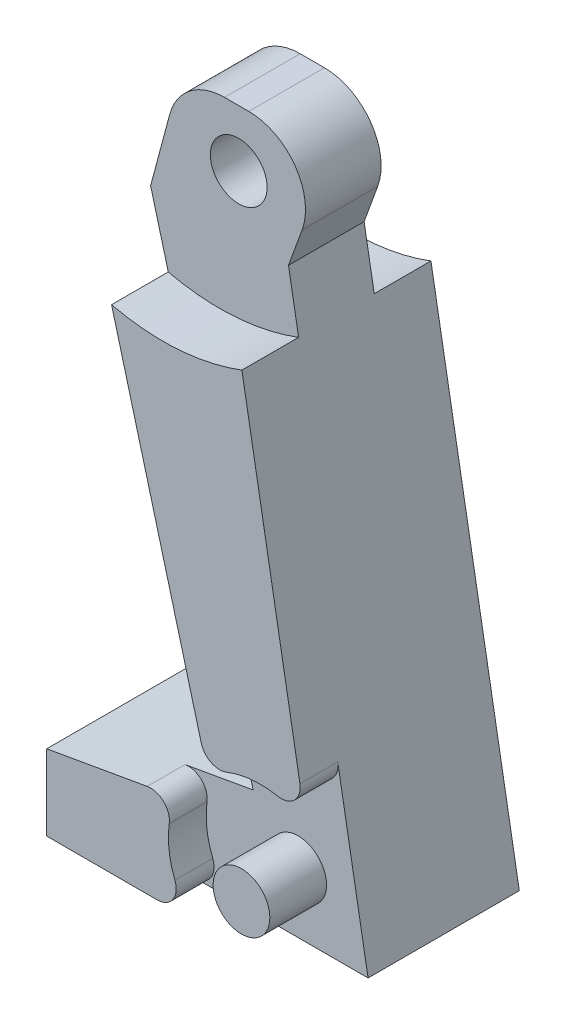
from build123d import *

# Parameters (mm, degrees)
BOSS_EXTRUDE1_DEPTH = 10
SKETCH2_W           = 14
SKETCH2_H           = 30
BOSS_EXTRUDE2_DEPTH = 30
BOSS_EXTRUDE4_DEPTH = 5
SKETCH5_W           = 6
SKETCH5_H           = 7
BOSS_EXTRUDE5_DEPTH = 6
SKETCH6_W           = 15
SKETCH6_H           = 15
BOSS_EXTRUDE6_DEPTH = 14
SKETCH7_R           = 1
CUT_EXTRUDE1_DEPTH  = 2
FILLET1_R           = 1
SKETCH8_R           = 1.5
SKETCH8_W           = 21.297654542
SKETCH8_H           = 29.54423259
CUT_EXTRUDE2_DEPTH  = 10
SKETCH9_W           = 4
SKETCH9_H           = 12
CUT_EXTRUDE3_DEPTH  = 7.5
SKETCH11_R          = 1.5
SKETCH11_W          = 46.682021109
SKETCH11_H          = 78.101327177
CUT_EXTRUDE6_DEPTH  = 50
SKETCH12_W          = 25.193851166
SKETCH12_H          = 16.960566472
CUT_EXTRUDE7_DEPTH  = 20
FILLET2_R           = 3
SKETCH13_W          = 3
SKETCH13_H          = 6
CUT_EXTRUDE8_DEPTH  = 20
SKETCH14_R          = 11.800022464
CUT_EXTRUDE9_DEPTH  = 3
SKETCH15_R          = 1.5
BOSS_EXTRUDE7_DEPTH = 1
SKETCH16_R          = 4.865347009
SKETCH16_R_2        = 1.5
CUT_EXTRUDE10_DEPTH = 2
FILLET5_R           = 1


with BuildPart() as part:
    # Sketch1 → Boss-Extrude1 (new body)
    with BuildSketch(Plane.XY):
        Polygon((0, 0), (15, 0), (9.79055467, 29.54423259), (20.05115897, 57.735011214), (10.05115897, 57.735011214), (2.497462604, 29.54423259), (8.920552671, 5.572934119), (0, 4), align=None)
    boss_extrude1 = extrude(amount=BOSS_EXTRUDE1_DEPTH)

    # Sketch2 → Boss-Extrude2 (add)
    with BuildSketch(Plane.XY.offset(10)):
        with Locations((15.05115897, 72.735011214)):
            Rectangle(SKETCH2_W, SKETCH2_H)
    extrude(amount=-BOSS_EXTRUDE2_DEPTH)

    # Sketch4 → Boss-Extrude4 (add)
    with BuildSketch(Plane.XY.offset(10)):
        Polygon((15.05115897, 84.235011214), (30.372047832, 71.37925902), (30.372047832, 56.37925902), (27.30787006, 56.37925902), (27.30787006, 68.950409459), (15.05115897, 79.235011214), align=None)
    boss_extrude4 = extrude(amount=BOSS_EXTRUDE4_DEPTH)

    # Mirror1: Boss-Extrude1, Boss-Extrude4 across plane
    add(boss_extrude1.mirror(Plane.XY.offset(-5)))
    add(boss_extrude4.mirror(Plane.XY.offset(-5)))

    # Sketch5 → Boss-Extrude5 (add)
    with BuildSketch(Plane(origin=(0, 87.735011214, 0), x_dir=(1, 0, 0), z_dir=(0, 1, 0))):
        with Locations((15.05115897, 5)):
            Rectangle(SKETCH5_W, SKETCH5_H)
    extrude(amount=BOSS_EXTRUDE5_DEPTH)

    # Sketch6 → Boss-Extrude6 (add)
    with BuildSketch(Plane(origin=(0, 93.735011214, 0), x_dir=(1, 0, 0), z_dir=(0, 1, 0))):
        with Locations((15.05115897, 5)):
            Rectangle(SKETCH6_W, SKETCH6_H)
    extrude(amount=BOSS_EXTRUDE6_DEPTH)

    # Sketch7 → Cut-Extrude1 (cut)
    with BuildSketch(Plane.ZY.offset(-7.55115897)):
        with Locations((-8.96, 103.735011214)):
            Circle(SKETCH7_R)
        with Locations(Location((-1.04, 103.735011214, 0), (0, 0, 180))):
            Circle(SKETCH7_R)
    extrude(amount=-CUT_EXTRUDE1_DEPTH, mode=Mode.SUBTRACT)

    # Fillet1
    fillet1_edges = [part.edges().sort_by_distance(p)[0] for p in [
        (18.55115897, 81.298162505, 10),
        (15.05115897, 81.735011214, 10),
        (15.05115897, 84.235011214, 12.5),
        (18.55115897, 76.298162505, 10),
        (15.05115897, 79.235011214, 12.5),
        (18.55115897, 81.298162505, -20),
        (18.55115897, 76.298162505, -20),
        (15.05115897, 81.735011214, -20),
        (15.05115897, 79.235011214, -22.5),
        (15.05115897, 84.235011214, -22.5),
    ]]
    fillet(fillet1_edges, radius=FILLET1_R)

    # Sketch8 → Cut-Extrude2 (cut)
    with BuildSketch(Plane(origin=(0, 0, -20), x_dir=(-1, 0, 0), z_dir=(0, 0, -1))):
        with Locations((-7.157843169, 32.54423259)):
            Circle(SKETCH8_R)
        with Locations((-4.351172729, 14.772116295)):
            Rectangle(SKETCH8_W, SKETCH8_H)
    extrude(amount=-CUT_EXTRUDE2_DEPTH, mode=Mode.SUBTRACT)

    # Sketch9 → Cut-Extrude3 (cut, symmetric)
    with BuildSketch(Plane.ZY.offset(-8.05115897)):
        with Locations((-15, 30.54423259)):
            Rectangle(SKETCH9_W, SKETCH9_H)
    extrude(amount=CUT_EXTRUDE3_DEPTH, both=True, mode=Mode.SUBTRACT)

    # Sketch11 → Cut-Extrude6 (cut, symmetric)
    with BuildSketch(Plane(origin=(0, 0, -20), x_dir=(-1, 0, 0), z_dir=(0, 0, -1))):
        with Locations(Location((-7.157843169, 32.54423259, 0), (0, 0, 180))):
            Circle(SKETCH11_R)
        with Locations((-27.446168312, 74.594896179)):
            Rectangle(SKETCH11_W, SKETCH11_H)
    extrude(amount=CUT_EXTRUDE6_DEPTH, both=True, mode=Mode.SUBTRACT)


with BuildPart() as cut_extrude6_piece_1:
    # of the separate pieces the step leaves, piece 1, a body of its own (cut_extrude6_pieces)
    add(part.part.solids().sort_by_distance((4.105157758, 35.54423259, 10))[0])

    # Fillet2
    fillet2_edges = [cut_extrude6_piece_1.edges().sort_by_distance(p)[0] for p in [
        (11.974376076, 35.54423259, 5),
        (4.105157758, 35.54423259, 5),
    ]]
    fillet(fillet2_edges, radius=FILLET2_R)

    # Sketch13 → Cut-Extrude8 (cut)
    with BuildSketch(Plane(origin=(0, 0, 0), x_dir=(0, 0, -1), z_dir=(1, 0, 0))):
        with Locations((-8.5, 32.54423259)):
            Rectangle(SKETCH13_W, SKETCH13_H)
        with Locations((-1.5, 32.54423259)):
            Rectangle(SKETCH13_W, SKETCH13_H)
    extrude(amount=CUT_EXTRUDE8_DEPTH, mode=Mode.SUBTRACT)

    # Sketch14 → Cut-Extrude9 (cut)
    with BuildSketch(Plane(origin=(0, 0, 0), x_dir=(-1, 0, 0), z_dir=(0, 0, -1))):
        with Locations((-6.144008637, 37.54423259)):
            Circle(SKETCH14_R)
    cut_extrude9 = extrude(amount=-CUT_EXTRUDE9_DEPTH, mode=Mode.SUBTRACT)

    # Mirror2: Cut-Extrude9 across plane
    add(cut_extrude9.mirror(Plane(origin=(0, 0, 5), x_dir=(1, 0, 0), z_dir=(0, 0, -1))), mode=Mode.SUBTRACT)

    # Sketch15 → Boss-Extrude7 (add)
    with BuildSketch(Plane.XY.offset(10)):
        with Locations((11.303234902, 3.163151803)):
            Circle(SKETCH15_R)
    extrude(amount=BOSS_EXTRUDE7_DEPTH)

    # Sketch16 → Cut-Extrude10 (cut)
    with BuildSketch(Plane.XY.offset(10)):
        with Locations((11.303234902, 3.163151803)):
            Circle(SKETCH16_R)
        with Locations((11.303234902, 3.163151803)):
            Circle(SKETCH16_R_2, mode=Mode.SUBTRACT)
    extrude(amount=-CUT_EXTRUDE10_DEPTH, mode=Mode.SUBTRACT)

    # Fillet5
    fillet5_edges = [cut_extrude6_piece_1.edges().sort_by_distance(p)[0] for p in [
        (6.891812395, 5.215212471, 9),
        (13.695196152, 7.399910339, 9),
        (8.500606317, 7.140195245, 9),
        (7.606469803, 0, 9),
    ]]
    fillet(fillet5_edges, radius=FILLET5_R)


with BuildPart() as cut_extrude6_piece_2:
    # of the separate pieces the step leaves, piece 2, a body of its own (cut_extrude6_pieces)
    add(part.part.solids().sort_by_distance((4.105157758, 35.54423259, -20))[0])


with BuildPart() as cut_extrude6_piece_3:
    # of the separate pieces the step leaves, piece 3, a body of its own (cut_extrude6_pieces)
    add(part.part.solids().sort_by_distance((4.105157758, 35.54423259, -10))[0])


with BuildPart() as cut_extrude7_tool:
    # Sketch12 → Cut-Extrude7 (new body)
    with BuildSketch(Plane(origin=(0, 0, -20), x_dir=(-1, 0, 0), z_dir=(0, 0, -1))):
        with Locations((-9.102890418, 33.861350945)):
            Rectangle(SKETCH12_W, SKETCH12_H)
    extrude(amount=-CUT_EXTRUDE7_DEPTH)


with BuildPart() as cut_extrude6_piece_2_1:
    add(cut_extrude6_piece_2.part)

    # Cut-Extrude7: cut by cut_extrude7_tool
    add(cut_extrude7_tool.part, mode=Mode.SUBTRACT)


with BuildPart() as cut_extrude6_piece_3_1:
    add(cut_extrude6_piece_3.part)

    # Cut-Extrude7: cut by cut_extrude7_tool
    add(cut_extrude7_tool.part, mode=Mode.SUBTRACT)


solid = cut_extrude6_piece_1.part
